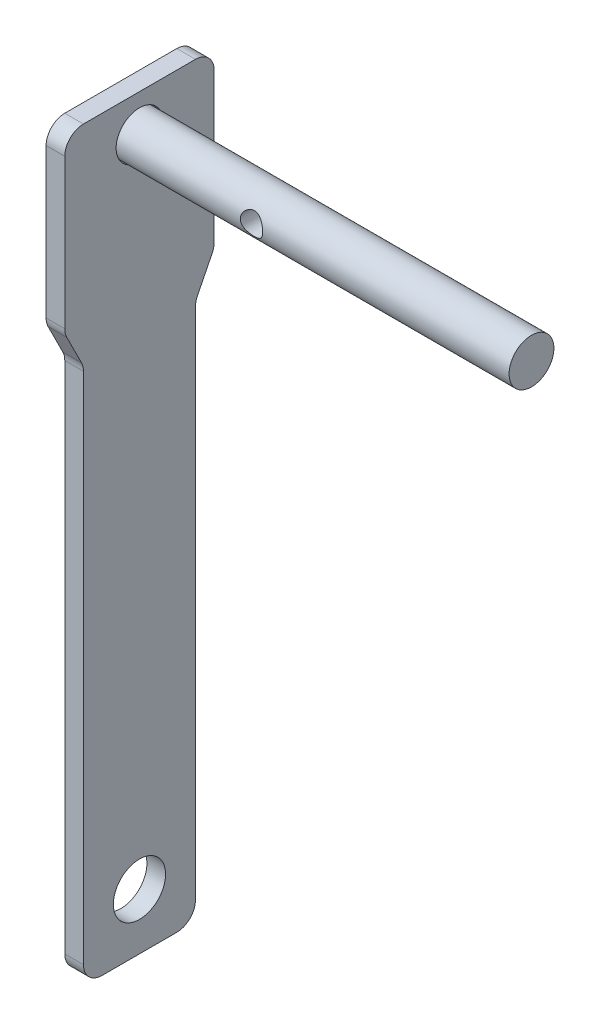
SolidWorks part; units mm, degrees
ref_plane "前视基准面" through (0, 0, 0) normal (0, 0, 1) x (1, 0, 0)
ref_plane "上视基准面" through (0, 0, 0) normal (0, 1, 0) x (1, 0, 0)
ref_plane "右视基准面" through (0, 0, 0) normal (1, 0, 0) x (0, 0, -1)
sketch "草图1" plane through (0, 0, 0) normal (0, 0, 1) x (1, 0, 0)
  line L2 (110, -190) -> (220, -190)
  point P7 (110, -190)
  dimension "D1" = 110
  dimension "D3" = 110
sweep "扫描1" add path "草图1" circular profile diameter 12 parameters "D3"=12
sketch "草图4" plane through (0, 0, 0) normal (0, 0, 1) x (1, 0, 0)
  line L0 (110, -190) -> (186.7447, -190) construction
  line L1 (110, -184) -> (110, -196) construction
  line L2 (220, -196) -> (220, -184) construction
  circle A0 centre (151, -190) radius 3
  dimension "D1" = 6
  dimension "D2" = 69
extrude "切除-拉伸2" cut sketch "草图4" against normal mid plane 80
sketch "草图6" plane through (110, 0, 0) normal (-1, 0, 0) x (0, 0, 1)
  line L0 (-19.4721, -227.2361) -> (-15.5279, -235.1246)
  line L1 (-15, -180) -> (15, -180)
  line L2 (-20, -185) -> (-20, -225)
  line L3 (-15, -380) -> (15, -380)
  line L4 (20, -185) -> (20, -225)
  line L5 (-15, -237.3607) -> (-15, -380)
  line L6 (19.4721, -227.2361) -> (15.5279, -235.1246)
  line L7 (15, -237.3607) -> (15, -380)
  circle A0 centre (0, -190) radius 6 construction
  arc A1 (15, -180) -> (20, -185) centre (15, -185) cw
  arc A2 (-15, -180) -> (-20, -185) centre (-15, -185) ccw
  circle A5 centre (0, -365) radius 7
  circle A6 centre (0, -190) radius 6.25
  arc A7 (19.4721, -227.2361) -> (20, -225) centre (15, -225) ccw
  arc A8 (15.5279, -235.1246) -> (15, -237.3607) centre (20, -237.3607) ccw
  arc A9 (-15.5279, -235.1246) -> (-15, -237.3607) centre (-20, -237.3607) cw
  arc A10 (-19.4721, -227.2361) -> (-20, -225) centre (-15, -225) cw
  point P8 (20, -180)
  point P11 (-20, -180)
  point P12 (20, -226.1803)
  point P23 (15, -236.1803)
  point P31 (-15, -236.1803)
  point P34 (-20, -226.1803)
  dimension "D2" = 20
  dimension "D3" = 10
  dimension "D4" = 5
  dimension "D6" = 5
  dimension "D7" = 14
  dimension "D9" = 20
  dimension "D10" = 12.5
  dimension "D1" = 40
  dimension "D5" = 200
  dimension "D8" = 15
  dimension "D11" = 5
  dimension "D12" = 5
  dimension "D13" = 10
  dimension "D14" = 10
  dimension "D15" = 45
extrude "凸台-拉伸2" add sketch "草图6" against normal blind 5 separate body
fillet "圆角1" radius 5 2 edges at (112.5, -380, -15) (112.5, -380, 15)
